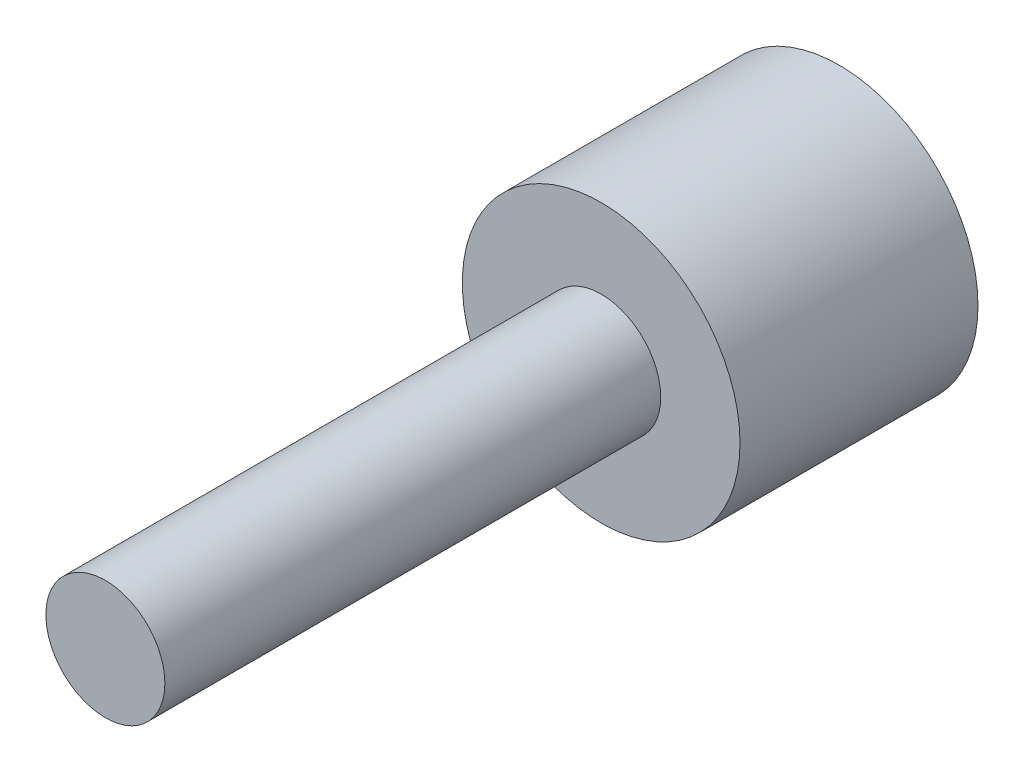
SolidWorks part; units mm, degrees
ref_plane "前视基准面" through (0, 0, 0) normal (0, 0, 1) x (1, 0, 0)
ref_plane "上视基准面" through (0, 0, 0) normal (0, 1, 0) x (1, 0, 0)
ref_plane "右视基准面" through (0, 0, 0) normal (1, 0, 0) x (0, 0, -1)
sketch "草图1" plane through (0, 0, 0) normal (0, 0, 1) x (1, 0, 0)
  circle A0 centre (0, 0) radius 7
  dimension "D1" = 14
extrude "凸台-拉伸1" add sketch "草图1" along normal blind 12
sketch "草图2" plane through (0, 0, 12) normal (0, 0, 1) x (1, 0, 0)
  circle A1 centre (0, 0) radius 3
  dimension "D1" = 6
extrude "凸台-拉伸2" add sketch "草图2" along normal blind 25
